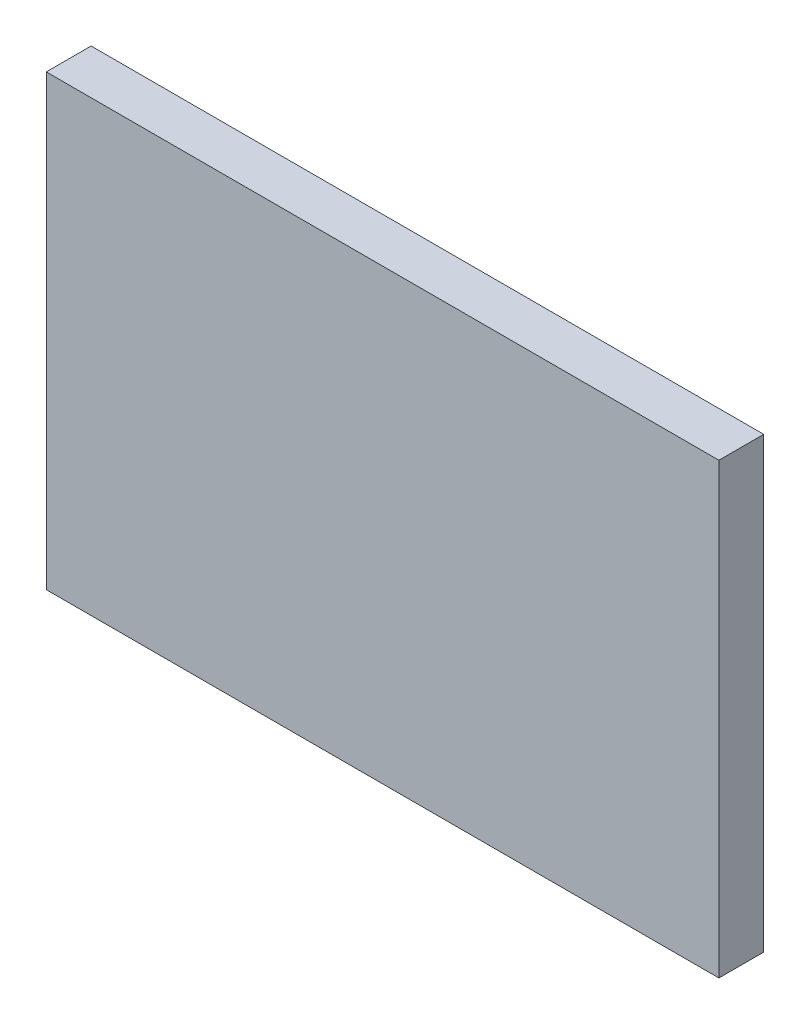
from build123d import *

# Parameters (mm, degrees)
SKETCH1_W           = 300
SKETCH1_H           = 200
BOSS_EXTRUDE1_DEPTH = 20
SKETCH2_W           = 270
SKETCH2_H           = 160
CUT_EXTRUDE1_DEPTH  = 10
SKETCH3_R           = 30
CUT_EXTRUDE2_DEPTH  = 6


with BuildPart() as part:
    # Sketch1 → Boss-Extrude1 (new body)
    with BuildSketch(Plane.XY):
        Rectangle(SKETCH1_W, SKETCH1_H)
    extrude(amount=BOSS_EXTRUDE1_DEPTH)

    # Sketch2 → Cut-Extrude1 (cut)
    with BuildSketch(Plane(origin=(0, 0, 0), x_dir=(-1, 0, 0), z_dir=(0, 0, -1))):
        Rectangle(SKETCH2_W, SKETCH2_H)
    extrude(amount=-CUT_EXTRUDE1_DEPTH, mode=Mode.SUBTRACT)

    # Sketch3 → Cut-Extrude2 (cut)
    with BuildSketch(Plane(origin=(0, 0, 10), x_dir=(-1, 0, 0), z_dir=(0, 0, -1))):
        Circle(SKETCH3_R)
    extrude(amount=-CUT_EXTRUDE2_DEPTH, mode=Mode.SUBTRACT)


solid = part.part
